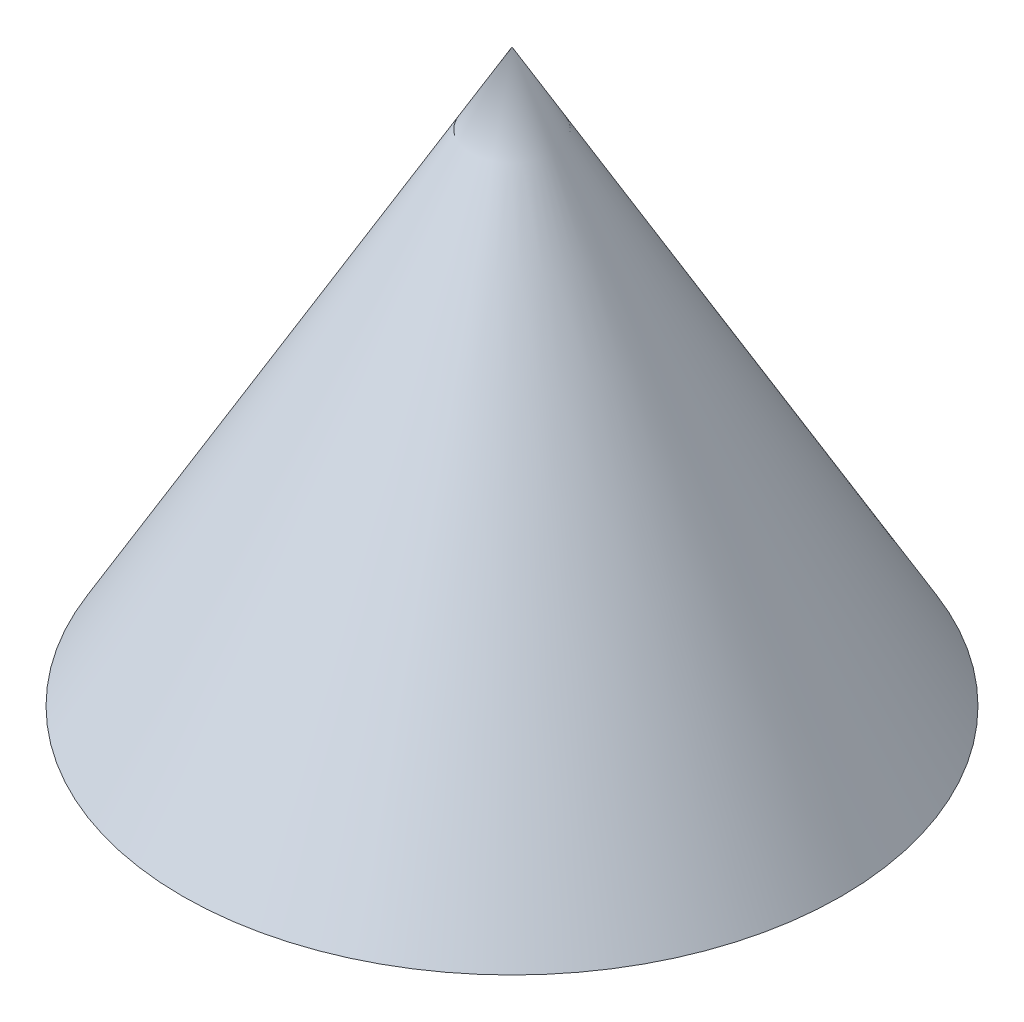
SolidWorks part; units mm, degrees
ref_plane "前视基准面" through (0, 0, 0) normal (0, 0, 1) x (1, 0, 0)
ref_plane "上视基准面" through (0, 0, 0) normal (0, 1, 0) x (1, 0, 0)
ref_plane "右视基准面" through (0, 0, 0) normal (1, 0, 0) x (0, 0, -1)
sketch "草图1" plane through (0, 0, 0) normal (0, 0, 1) x (1, 0, 0)
  line L0 (0, 0) -> (57.735, 0)
  line L1 (57.735, 0) -> (0, 100)
  line L2 (0, 100) -> (0, 0)
  dimension "D1" = 30
  dimension "D2" = 100
revolve "旋转1" add sketch "草图1" angle 360 about L2
